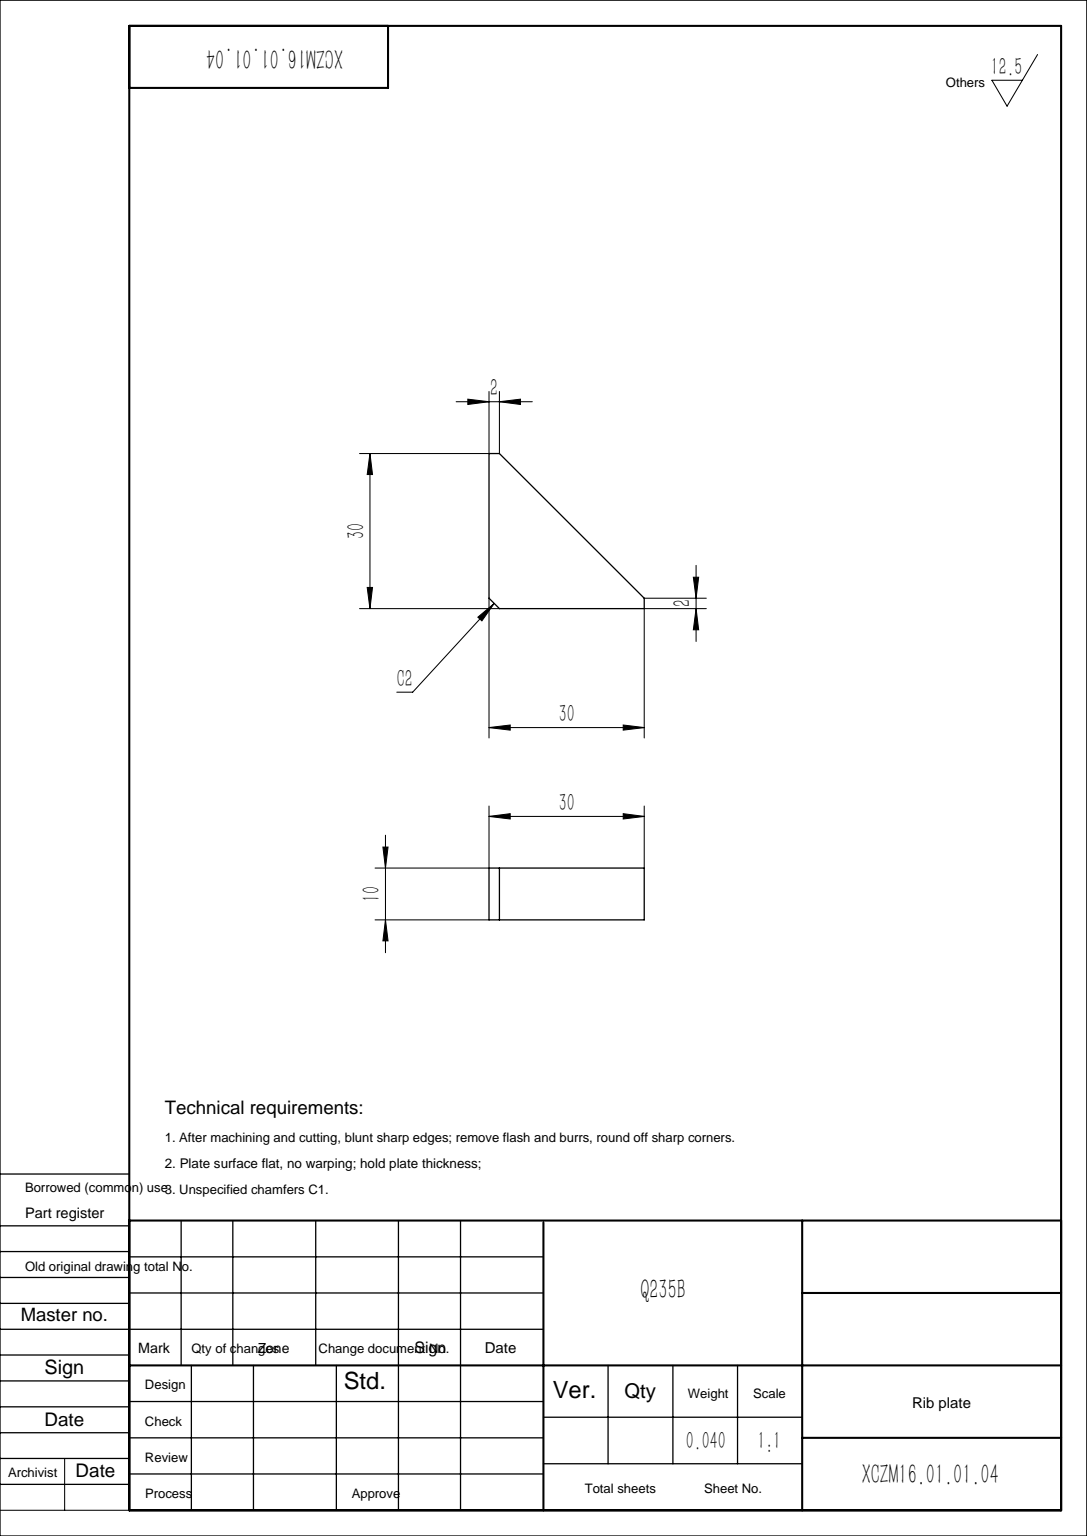
SolidWorks part; units mm, degrees
material "XRAAT"
ref_plane "前视基准面" through (0, 0, 0) normal (0, 0, 1) x (1, 0, 0)
ref_plane "上视基准面" through (0, 0, 0) normal (0, 1, 0) x (1, 0, 0)
ref_plane "右视基准面" through (0, 0, 0) normal (1, 0, 0) x (0, 0, -1)
sketch "草图1" plane through (0, 0, 0) normal (0, 0, 1) x (1, 0, 0)
  line L0 (0, 30) -> (0, 0)
  line L1 (0, 0) -> (30, 0)
  line L2 (30, 0) -> (30, 2)
  line L3 (30, 2) -> (2, 30)
  line L4 (2, 30) -> (0, 30)
  dimension "D1" = 30
  dimension "D2" = 2
extrude "凸台-拉伸1" add sketch "草图1" along normal blind 10
chamfer "倒角1" distance 2 angle 45 1 edges at (0, 0, 5)
